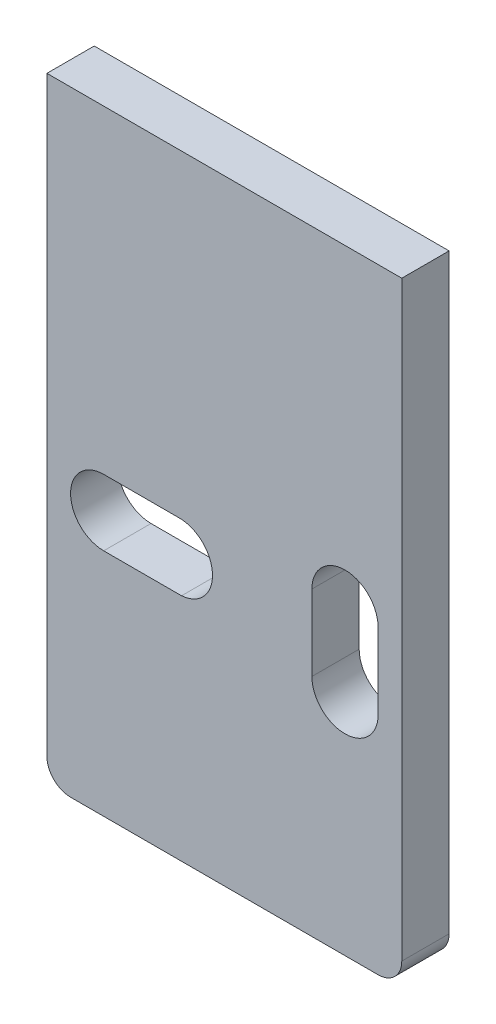
SolidWorks part; units mm, degrees
ref_plane "前视基准面" through (0, 0, 0) normal (0, 0, 1) x (1, 0, 0)
ref_plane "上视基准面" through (0, 0, 0) normal (0, 1, 0) x (1, 0, 0)
ref_plane "右视基准面" through (0, 0, 0) normal (1, 0, 0) x (0, 0, -1)
sketch "草图1" plane through (0, 0, 0) normal (0, 0, 1) x (1, 0, 0)
  line L1 (-37.5, 54.4) -> (37.5, 54.4)
  line L2 (-37.5, 54.4) -> (-37.5, -70.6)
  line L3 (-32.5, -75.6) -> (32.5, -75.6)
  line L4 (37.5, 54.4) -> (37.5, -70.6)
  line L6 (-9.0346, -27) -> (-9.0293, -26.9842) construction
  line L8 (18.5, -12) -> (18.5, -28)
  line L10 (32.5, -12) -> (32.5, -28)
  line L11 (-25.5, -13) -> (-9.5, -13)
  line L13 (-25.5, -27) -> (-9.0346, -27)
  arc A0 (-25.5, -13) -> (-25.5, -27) centre (-25.5, -20) ccw
  arc A1 (-9.0293, -26.9842) -> (-9.5, -13) centre (-9.5, -20) ccw
  arc A2 (32.5, -12) -> (18.5, -12) centre (25.5, -12) ccw
  arc A3 (18.5, -28) -> (32.5, -28) centre (25.5, -28) ccw
  arc A4 (32.5, -75.6) -> (37.5, -70.6) centre (32.5, -70.6) ccw
  arc A5 (-37.5, -70.6) -> (-32.5, -75.6) centre (-32.5, -70.6) ccw
  point P0 (0, 0)
  point P14 (37.5, -75.6)
  point P20 (0, 0)
  point P22 (18.5, -20)
  dimension "D9" = 12
  dimension "D10" = 5
  dimension "D1" = 75
  dimension "D2" = 130
  dimension "D3" = 14
  dimension "D4" = 16
  dimension "D6" = 5
  dimension "D7" = 14
  dimension "D8" = 16
  dimension "D11" = 55.6
extrude "凸台-拉伸1" add sketch "草图1" along normal blind 10 contours L2 A5 L3 A4 L4 L1 L6 L13 A0 L11 A1 A3 L8 A2 L10
